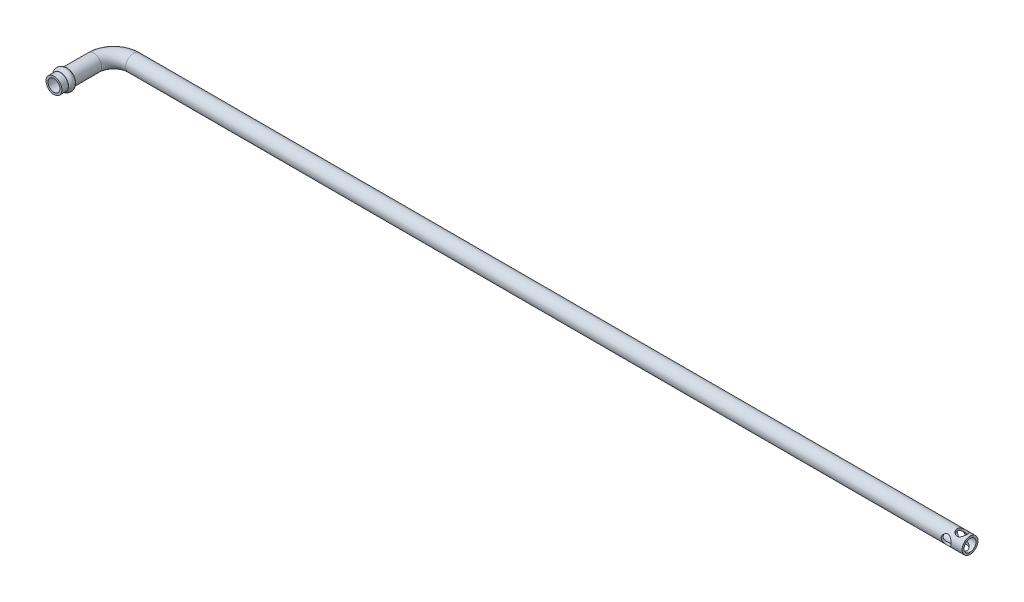
SolidWorks part; units mm, degrees
material "10#"
ref_plane "Front Plane" through (0, 0, 0) normal (0, 0, 1) x (1, 0, 0)
ref_plane "Top Plane" through (0, 0, 0) normal (0, 1, 0) x (1, 0, 0)
ref_plane "Right Plane" through (0, 0, 0) normal (1, 0, 0) x (0, 0, -1)
sketch "Sketch1" plane through (0, 0, 0) normal (0, 0, 1) x (1, 0, 0)
  circle A0 centre (0, 0) radius 3
  circle A1 centre (0, 0) radius 4
  dimension "D1" = 8
  dimension "D2" = 1
sketch "Sketch2" plane through (0, 0, 0) normal (0, 1, 0) x (1, 0, 0)
  line L0 (0, 0) -> (0, 20)
  line L1 (10, 30) -> (430, 30)
  arc A0 (0, 20) -> (10, 30) centre (10, 20) cw
  dimension "D1" = 10
  dimension "D2" = 30
  dimension "D3" = 430
sweep "Sweep1" add profiles "Sketch1" path "Sketch2"
sketch "Sketch3" plane through (0, 0, 0) normal (0, 1, 0) x (1, 0, 0)
  line L0 (-4, 0) -> (4, 0) construction
  line L2 (-4, 20) -> (-4, 0) construction
  line L3 (-4, 6.7321) -> (-4, 3.2679)
  line L4 (0, 0) -> (0, 9.9491) construction
  arc A0 (-4, 6.7321) -> (-4, 3.2679) centre (-3, 5) ccw
  dimension "D2" = 2
  dimension "D1" = 5
  dimension "D3" = 3
revolve "Revolve1" add sketch "Sketch3" angle 360 about L4
fillet "Fillet1" radius 0.1 2 edges at (4, 0, -3.2679) (4, 0, -6.7321)
sketch "Sketch4" plane through (0, 0, 0) normal (0, 1, 0) x (1, 0, 0)
  line L0 (430, 26) -> (430, 34) construction
  circle A0 centre (426, 30) radius 2.5
  dimension "D1" = 5
  dimension "D2" = 4
  dimension "D3" = 4
extrude "Cut-Extrude1" cut sketch "Sketch4" against normal through all both and the other way through all
sketch "Sketch5" plane through (0, 0, 0) normal (0, 0, 1) x (1, 0, 0)
  line L0 (430, -4) -> (430, 4) construction
  circle A0 centre (422, 0) radius 2.5
  dimension "D1" = 5
  dimension "D2" = 8
extrude "Cut-Extrude2" cut sketch "Sketch5" against normal through all both and the other way through all
